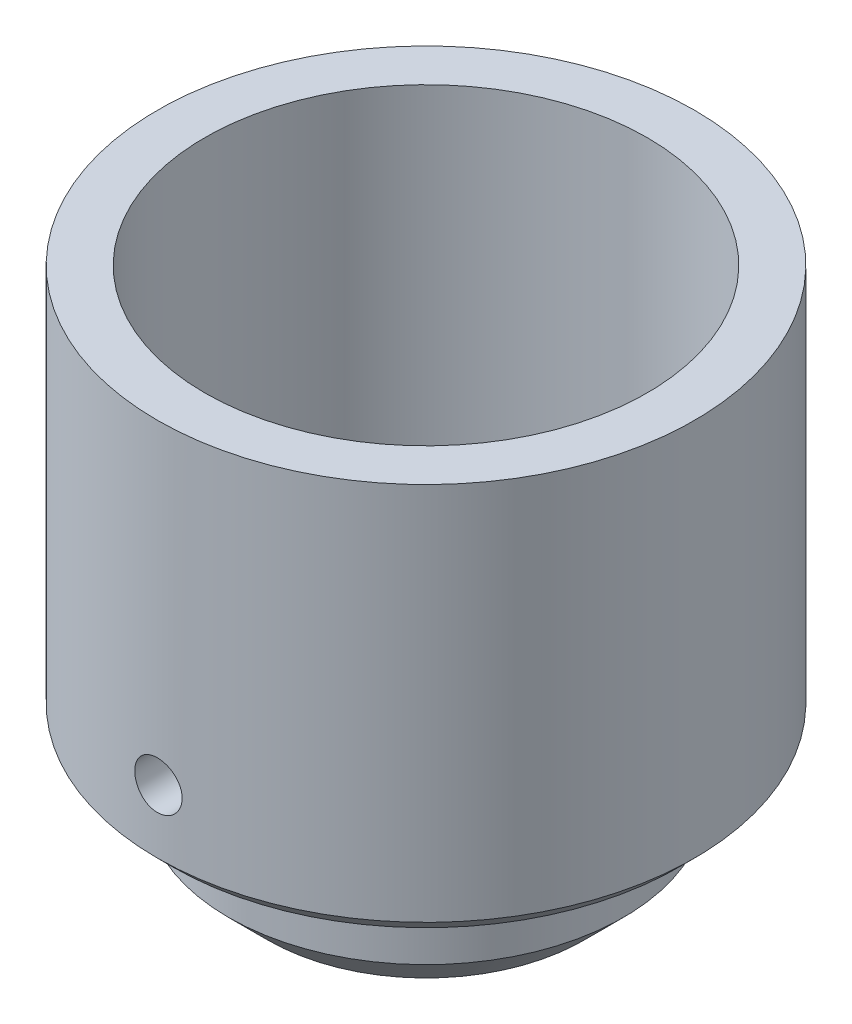
SolidWorks part; units mm, degrees
ref_plane "Front Plane" through (0, 0, 0) normal (0, 0, 1) x (1, 0, 0)
ref_plane "Top Plane" through (0, 0, 0) normal (0, 1, 0) x (1, 0, 0)
ref_plane "Right Plane" through (0, 0, 0) normal (1, 0, 0) x (0, 0, -1)
other "Configuration Table"
sketch "Sketch1" plane through (0, 0, 0) normal (0, 0, 1) x (1, 0, 0)
  line L0 (0, 19.3805) -> (0, -24.3556) construction
  line L1 (0, 0) -> (-10, 0)
  line L2 (-10, 0) -> (-12.5, 2.5)
  line L3 (-12.5, 2.5) -> (-12.5, 7)
  line L4 (-12.5, 7) -> (-16, 7)
  line L5 (-17, 8) -> (-17, 32)
  line L6 (-17, 32) -> (-14, 32)
  line L7 (-14, 32) -> (-14, 10)
  line L8 (-14, 10) -> (0, 10)
  line L9 (-16, 7) -> (-17, 8)
  line L10 (0, 10) -> (0, 0)
  point P8 (-17, 7)
  dimension "D1" = 14
  dimension "D2" = 17
  dimension "D3" = 12.5
  dimension "D4" = 2.5
  dimension "D5" = 135
  dimension "D6" = 22
  dimension "D7" = 32
  dimension "D8" = 7
revolve "Revolve1" add sketch "Sketch1" angle 360 about L0
sketch "Sketch2" plane through (0, 10, 0) normal (0, 1, 0) x (1, 0, 0)
  point P0 (0, 0)
hole_wizard "M6 Tapped Hole1" positions "Sketch2" profile "Sketch3" tap size "M6" standard "GB"
sketch "Sketch3" plane through (0, 10, 0) normal (1, 0, 0) x (0, 0, 1)
  line L0 (0, 0) -> (0, 6.5022)
  line L1 (0, 6.5022) -> (2.5, 5)
  line L2 (2.5, 5) -> (2.5, 0)
  line L5 (2.5, 0) -> (0, 0)
  line L10 (0, 6.5022) -> (-2.5, 5) construction
  line L11 (0, -6.35) -> (0, 107.95) construction
  dimension "螺纹孔钻头直径" = 5
  dimension "螺纹孔钻头深度" = 5
  dimension "导头角度" = 118
cosmetic thread "Cosmetic Thread1" parameters "D1"=12, "D2"=6
sketch "Sketch4" plane through (0, 0, 0) normal (0, 0, 1) x (1, 0, 0)
  line L0 (0, 0) -> (0, 35.9742) construction
  line L1 (17, 32) -> (-17, 32) construction
  circle A0 centre (0, 12) radius 1.5
  dimension "D1" = 3
  dimension "D2" = 20
extrude "Cut-Extrude1" cut sketch "Sketch4" against normal mid plane 70
